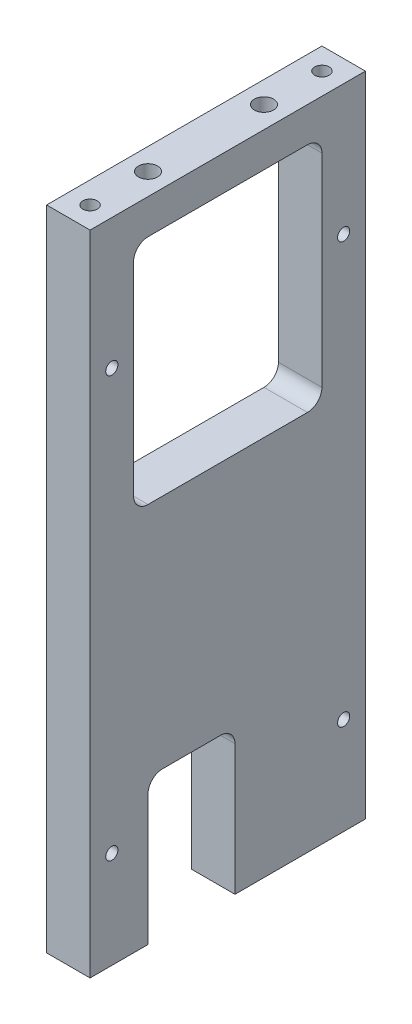
SolidWorks part; units mm, degrees
material "A6061"
ref_plane "Front Plane" through (0, 0, 0) normal (0, 0, 1) x (1, 0, 0)
ref_plane "Top Plane" through (0, 0, 0) normal (0, 1, 0) x (1, 0, 0)
ref_plane "Right Plane" through (0, 0, 0) normal (1, 0, 0) x (0, 0, -1)
sketch "Sketch1" plane through (0, 0, 0) normal (1, 0, 0) x (0, 0, -1)
  line L1 (-47.5, -111.75) -> (47.5, -111.75)
  line L2 (-47.5, -111.75) -> (-47.5, 111.75)
  line L3 (-47.5, 111.75) -> (47.5, 111.75)
  line L4 (47.5, -111.75) -> (47.5, 111.75)
  line L5 (-47.5, -111.75) -> (47.5, 111.75) construction
  line L6 (-47.5, 111.75) -> (47.5, -111.75) construction
  point P0 (0, 0)
  dimension "D1" = 95
  dimension "D2" = 223.5
extrude "Boss-Extrude1" add sketch "Sketch1" along normal blind 15
sketch "Sketch2" plane through (0, 0, 0) normal (-1, 0, 0) x (0, 0, 1)
  line L0 (-47.5, -111.75) -> (-47.5, 111.75) construction
  line L1 (47.5, -111.75) -> (-47.5, -111.75) construction
  line L2 (22.5, -61.75) -> (2.5, -61.75)
  line L3 (27.5, -66.75) -> (27.5, -111.75)
  line L4 (27.5, -111.75) -> (-2.5, -111.75)
  line L5 (-2.5, -66.75) -> (-2.5, -111.75)
  line L6 (27.5, -61.75) -> (-2.5, -111.75) construction
  line L7 (27.5, -111.75) -> (-2.5, -61.75) construction
  line L8 (47.5, 111.75) -> (47.5, -111.75) construction
  line L9 (-27.5, 19.75) -> (27.5, 19.75)
  line L10 (-32.5, 24.75) -> (-32.5, 94.75)
  line L11 (-27.5, 99.75) -> (27.5, 99.75)
  line L12 (32.5, 24.75) -> (32.5, 94.75)
  line L13 (-32.5, 19.75) -> (32.5, 99.75) construction
  line L14 (-32.5, 99.75) -> (32.5, 19.75) construction
  line L15 (-47.5, 111.75) -> (47.5, 111.75) construction
  arc A0 (22.5, -61.75) -> (27.5, -66.75) centre (22.5, -66.75) cw
  arc A1 (2.5, -61.75) -> (-2.5, -66.75) centre (2.5, -66.75) ccw
  arc A2 (27.5, 19.75) -> (32.5, 24.75) centre (27.5, 24.75) ccw
  arc A3 (-27.5, 19.75) -> (-32.5, 24.75) centre (-27.5, 24.75) cw
  arc A4 (27.5, 99.75) -> (32.5, 94.75) centre (27.5, 94.75) cw
  arc A5 (-32.5, 94.75) -> (-27.5, 99.75) centre (-27.5, 94.75) cw
  point P3 (12.5, -86.75)
  point P16 (0, 59.75)
  dimension "D3" = 5
  dimension "D7" = 5
  dimension "D1" = 30
  dimension "D2" = 50
  dimension "D4" = 15
  dimension "D5" = 12
  dimension "D6" = 80
  dimension "D8" = 15
  dimension "D9" = 20
extrude "Cut-Extrude1" cut sketch "Sketch2" against normal through all
hole_wizard "M6 Clearance Hole1" positions "Sketch6" profile "Sketch7" hole size "M6" standard "GB"
sketch "Sketch6" plane through (0, 111.75, 0) normal (0, 1, 0) x (1, 0, 0)
  line L0 (0, 0) -> (15, 0) construction
  line L1 (15, 47.5) -> (15, -47.5) construction
  line L3 (7.5, 47.5) -> (7.5, -47.5) construction
  line L4 (15, 47.5) -> (0, 47.5) construction
  line L5 (15, -47.5) -> (0, -47.5) construction
  point P16 (7.5, 20)
  point P18 (7.5, -20)
  dimension "D1" = 40
sketch "Sketch7" plane through (7.5, 111.75, 20) normal (1, 0, 0) x (0, 0, 1)
  line L0 (0, 0) -> (0, 21.7328)
  line L1 (0, 21.7328) -> (3.3, 19.75)
  line L2 (3.3, 19.75) -> (3.3, 0)
  line L5 (3.3, 0) -> (0, 0)
  line L10 (0, 21.7328) -> (-3.3, 19.75) construction
  line L11 (0, -6.35) -> (0, 107.95) construction
  dimension "孔直径" = 6.6
  dimension "孔深度" = 19.75
  dimension "导头角度" = 118
hole_wizard "M6 Tapped Hole1" positions "Sketch8" profile "Sketch9" tap size "M6" standard "GB"
sketch "Sketch8" plane through (0, -111.75, 0) normal (0, -1, 0) x (-1, 0, 0)
  line L0 (0, 0) -> (-15, 0) construction
  line L3 (-7.5, 47.5) -> (-7.5, -47.5) construction
  line L4 (-15, 47.5) -> (0, 47.5) construction
  line L5 (-15, -47.5) -> (0, -47.5) construction
  line L6 (-15, 2.5) -> (-15, 47.5) construction
  point P16 (-7.5, 40)
  point P18 (-7.5, -40)
  dimension "D1" = 80
sketch "Sketch9" plane through (7.5, -111.75, 40) normal (1, 0, 0) x (0, 0, -1)
  line L0 (0, 0) -> (0, 16.5022)
  line L1 (0, 16.5022) -> (2.5, 15)
  line L2 (2.5, 15) -> (2.5, 0)
  line L5 (2.5, 0) -> (0, 0)
  line L10 (0, 16.5022) -> (-2.5, 15) construction
  line L11 (0, -6.35) -> (0, 107.95) construction
  dimension "螺纹孔钻头直径" = 5
  dimension "螺纹孔钻头深度" = 15
  dimension "导头角度" = 118
hole_wizard "Ø5.0mm blind hole 1" positions "Sketch10" profile "Sketch11" hole size "Ø5.0" standard "GB"
sketch "Sketch10" plane through (0, -111.75, 0) normal (0, -1, 0) x (-1, 0, 0)
  line L0 (-7.5, 40) -> (-7.5, -40) construction
  point P7 (-7.5, 10)
  dimension "D1" = 10
sketch "Sketch11" plane through (7.5, -111.75, -10) normal (1, 0, 0) x (0, 0, -1)
  line L0 (0, 0) -> (0, 9.5022)
  line L1 (0, 9.5022) -> (2.5, 8)
  line L2 (2.5, 8) -> (2.5, 0)
  line L5 (2.5, 0) -> (0, 0)
  line L10 (0, 9.5022) -> (-2.5, 8) construction
  line L11 (0, -6.35) -> (0, 107.95) construction
  dimension "孔直径" = 5
  dimension "孔深度" = 8
  dimension "导头角度" = 118
hole_wizard "Ø5.0mm blind hole 2" positions "Sketch12" profile "Sketch13" hole size "Ø5.0" standard "GB"
sketch "Sketch12" plane through (0, 111.75, 0) normal (0, 1, 0) x (1, 0, 0)
  line L0 (0, 0) -> (15, 0) construction
  line L1 (15, 47.5) -> (15, -47.5) construction
  line L3 (7.5, 47.5) -> (7.5, -47.5) construction
  line L4 (15, 47.5) -> (0, 47.5) construction
  line L5 (15, -47.5) -> (0, -47.5) construction
  point P16 (7.5, 40)
  point P18 (7.5, -40)
  dimension "D1" = 80
sketch "Sketch13" plane through (7.5, 111.75, 40) normal (1, 0, 0) x (0, 0, 1)
  line L0 (0, 0) -> (0, 9.5022)
  line L1 (0, 9.5022) -> (2.5, 8)
  line L2 (2.5, 8) -> (2.5, 0)
  line L5 (2.5, 0) -> (0, 0)
  line L10 (0, 9.5022) -> (-2.5, 8) construction
  line L11 (0, -6.35) -> (0, 107.95) construction
  dimension "孔直径" = 5
  dimension "孔深度" = 8
  dimension "导头角度" = 118
hole_wizard "M5 Tapped Hole1" positions "Sketch16" profile "Sketch17" tap size "M5" standard "GB"
sketch "Sketch16" plane through (15, 0, 0) normal (1, 0, 0) x (0, 0, -1)
  point P0 (40, 66.75)
  point P3 (-40, 66.75)
  point P6 (40, -78.25)
  point P9 (-40, -78.25)
sketch "Sketch17" plane through (15, 66.75, -40) normal (0, 1, 0) x (0, 0, -1)
  line L0 (0, 0) -> (0, 13.6618)
  line L1 (0, 13.6618) -> (2.1, 12.4)
  line L2 (2.1, 12.4) -> (2.1, 0)
  line L5 (2.1, 0) -> (0, 0)
  line L10 (0, 13.6618) -> (-2.1, 12.4) construction
  line L11 (0, -6.35) -> (0, 107.95) construction
  dimension "螺纹孔钻头直径" = 4.2
  dimension "螺纹孔钻头深度" = 12.4
  dimension "导头角度" = 118
